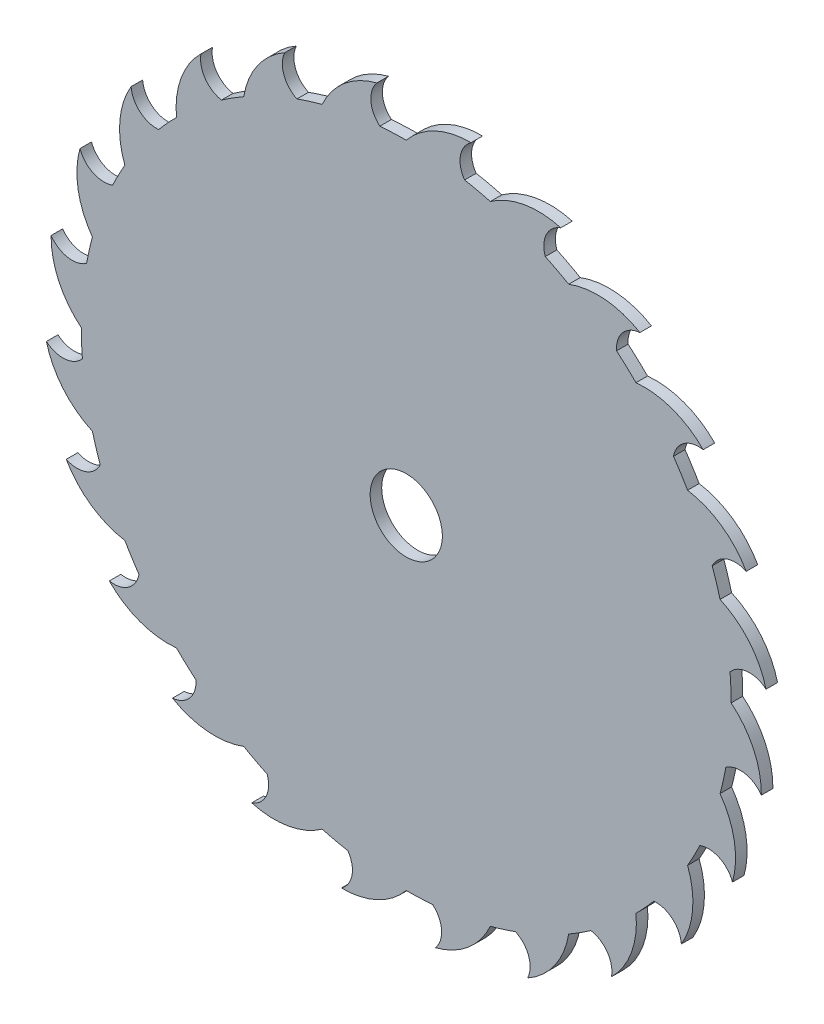
SolidWorks part; units mm, degrees
ref_plane "Front Plane" through (0, 0, 0) normal (0, 0, 1) x (1, 0, 0)
ref_plane "Top Plane" through (0, 0, 0) normal (0, 1, 0) x (1, 0, 0)
ref_plane "Right Plane" through (0, 0, 0) normal (1, 0, 0) x (0, 0, -1)
other "Configuration Table"
ref_plane "Plane1" through (0, 0, 4) normal (0, 0, 1) x (1, 0, 0)
sketch "Sketch1" plane through (0, 0, 4) normal (0, 0, 1) x (1, 0, 0)
  arc A0 (22.4405, 122.9692) -> (0, 112.5) centre (22.1215, 94.3681) ccw
  arc A1 (0, 112.5) -> (-9.1359, 112.1284) centre (0, 0) ccw
  arc A2 (-9.1359, 112.1284) -> (-10.151, 124.5872) centre (-3.4141, 118.8653) cw
  arc A3 (-10.151, 124.5872) -> (-29.1171, 108.6667) centre (-3.0565, 96.878) ccw
  arc A4 (-29.1171, 108.6667) -> (-37.8455, 105.9432) centre (0, 0) ccw
  arc A5 (-37.8455, 105.9432) -> (-42.0506, 117.7147) centre (-34.0623, 113.9315) cw
  arc A6 (-42.0506, 117.7147) -> (-56.25, 97.4279) centre (-28.0263, 92.7859) ccw
  arc A7 (-56.25, 97.4279) -> (-63.9761, 92.5381) centre (0, 0) ccw
  arc A8 (-63.9761, 92.5381) -> (-71.0846, 102.8202) centre (-62.3893, 101.2334) cw
  arc A9 (-71.0846, 102.8202) -> (-79.5495, 79.5495) centre (-51.0861, 82.3706) ccw
  arc A10 (-79.5495, 79.5495) -> (-85.7468, 72.8267) centre (0, 0) ccw
  arc A11 (-85.7468, 72.8267) -> (-95.2742, 80.9186) centre (-86.4646, 81.6364) cw
  arc A12 (-95.2742, 80.9186) -> (-97.4279, 56.25) centre (-70.6644, 66.3418) ccw
  arc A13 (-97.4279, 56.25) -> (-101.674, 48.1523) centre (0, 0) ccw
  arc A14 (-101.674, 48.1523) -> (-112.9711, 53.5026) centre (-104.6474, 56.476) cw
  arc A15 (-112.9711, 53.5026) -> (-108.6667, 29.1171) centre (-85.4271, 45.792) ccw
  arc A16 (-108.6667, 29.1171) -> (-110.6723, 20.1964) centre (0, 0) ccw
  arc A17 (-110.6723, 20.1964) -> (-122.9692, 22.4405) centre (-115.6987, 27.4669) cw
  arc A18 (-122.9692, 22.4405) -> (-112.5, 0) centre (-94.3681, 22.1215) ccw
  arc A19 (-112.5, 0) -> (-112.1284, -9.1359) centre (0, 0) ccw
  arc A20 (-112.1284, -9.1359) -> (-124.5872, -10.151) centre (-118.8653, -3.4141) cw
  arc A21 (-124.5872, -10.151) -> (-108.6667, -29.1171) centre (-96.878, -3.0565) ccw
  arc A22 (-108.6667, -29.1171) -> (-105.9432, -37.8455) centre (0, 0) ccw
  arc A23 (-105.9432, -37.8455) -> (-117.7147, -42.0506) centre (-113.9315, -34.0623) cw
  arc A24 (-117.7147, -42.0506) -> (-97.4279, -56.25) centre (-92.7859, -28.0263) ccw
  arc A25 (-97.4279, -56.25) -> (-92.5381, -63.9761) centre (0, 0) ccw
  arc A26 (-92.5381, -63.9761) -> (-102.8202, -71.0846) centre (-101.2334, -62.3893) cw
  arc A27 (-102.8202, -71.0846) -> (-79.5495, -79.5495) centre (-82.3706, -51.0861) ccw
  arc A28 (-79.5495, -79.5495) -> (-72.8267, -85.7468) centre (0, 0) ccw
  arc A29 (-72.8267, -85.7468) -> (-80.9186, -95.2742) centre (-81.6364, -86.4646) cw
  arc A30 (-80.9186, -95.2742) -> (-56.25, -97.4279) centre (-66.3418, -70.6644) ccw
  arc A31 (-56.25, -97.4279) -> (-48.1523, -101.674) centre (0, 0) ccw
  arc A32 (-48.1523, -101.674) -> (-53.5026, -112.9711) centre (-56.476, -104.6474) cw
  arc A33 (-53.5026, -112.9711) -> (-29.1171, -108.6667) centre (-45.792, -85.4271) ccw
  arc A34 (-29.1171, -108.6667) -> (-20.1964, -110.6723) centre (0, 0) ccw
  arc A35 (-20.1964, -110.6723) -> (-22.4405, -122.9692) centre (-27.4669, -115.6987) cw
  arc A36 (-22.4405, -122.9692) -> (0, -112.5) centre (-22.1215, -94.3681) ccw
  arc A37 (0, -112.5) -> (9.1359, -112.1284) centre (0, 0) ccw
  arc A38 (9.1359, -112.1284) -> (10.151, -124.5872) centre (3.4141, -118.8653) cw
  arc A39 (10.151, -124.5872) -> (29.1171, -108.6667) centre (3.0565, -96.878) ccw
  arc A40 (29.1171, -108.6667) -> (37.8455, -105.9432) centre (0, 0) ccw
  arc A41 (37.8455, -105.9432) -> (42.0506, -117.7147) centre (34.0623, -113.9315) cw
  arc A42 (42.0506, -117.7147) -> (56.25, -97.4279) centre (28.0263, -92.7859) ccw
  arc A43 (56.25, -97.4279) -> (63.9761, -92.5381) centre (0, 0) ccw
  arc A44 (63.9761, -92.5381) -> (71.0846, -102.8202) centre (62.3893, -101.2334) cw
  arc A45 (71.0846, -102.8202) -> (79.5495, -79.5495) centre (51.0861, -82.3706) ccw
  arc A46 (79.5495, -79.5495) -> (85.7468, -72.8267) centre (0, 0) ccw
  arc A47 (85.7468, -72.8267) -> (95.2742, -80.9186) centre (86.4646, -81.6364) cw
  arc A48 (95.2742, -80.9186) -> (97.4279, -56.25) centre (70.6644, -66.3418) ccw
  arc A49 (97.4279, -56.25) -> (101.674, -48.1523) centre (0, 0) ccw
  arc A50 (101.674, -48.1523) -> (112.9711, -53.5026) centre (104.6474, -56.476) cw
  arc A51 (112.9711, -53.5026) -> (108.6667, -29.1171) centre (85.4271, -45.792) ccw
  arc A52 (108.6667, -29.1171) -> (110.6723, -20.1964) centre (0, 0) ccw
  arc A53 (110.6723, -20.1964) -> (122.9692, -22.4405) centre (115.6987, -27.4669) cw
  arc A54 (122.9692, -22.4405) -> (112.5, 0) centre (94.3681, -22.1215) ccw
  arc A55 (112.5, 0) -> (112.1284, 9.1359) centre (0, 0) ccw
  arc A56 (112.1284, 9.1359) -> (124.5872, 10.151) centre (118.8653, 3.4141) cw
  arc A57 (124.5872, 10.151) -> (108.6667, 29.1171) centre (96.878, 3.0565) ccw
  arc A58 (108.6667, 29.1171) -> (105.9432, 37.8455) centre (0, 0) ccw
  arc A59 (105.9432, 37.8455) -> (117.7147, 42.0506) centre (113.9315, 34.0623) cw
  arc A60 (117.7147, 42.0506) -> (97.4279, 56.25) centre (92.7859, 28.0263) ccw
  arc A61 (97.4279, 56.25) -> (92.5381, 63.9761) centre (0, 0) ccw
  arc A62 (92.5381, 63.9761) -> (102.8202, 71.0846) centre (101.2334, 62.3893) cw
  arc A63 (102.8202, 71.0846) -> (79.5495, 79.5495) centre (82.3706, 51.0861) ccw
  arc A64 (79.5495, 79.5495) -> (72.8267, 85.7468) centre (0, 0) ccw
  arc A65 (72.8267, 85.7468) -> (80.9186, 95.2742) centre (81.6364, 86.4646) cw
  arc A66 (80.9186, 95.2742) -> (56.25, 97.4279) centre (66.3418, 70.6644) ccw
  arc A67 (56.25, 97.4279) -> (48.1523, 101.674) centre (0, 0) ccw
  arc A68 (48.1523, 101.674) -> (53.5026, 112.9711) centre (56.476, 104.6474) cw
  arc A69 (53.5026, 112.9711) -> (29.1171, 108.6667) centre (45.792, 85.4271) ccw
  arc A70 (29.1171, 108.6667) -> (20.1964, 110.6723) centre (0, 0) ccw
  arc A71 (20.1964, 110.6723) -> (22.4405, 122.9692) centre (27.4669, 115.6987) cw
  circle A72 centre (0, 0) radius 12.5
extrude "Boss-Extrude1" add sketch "Sketch1" against normal blind 4
